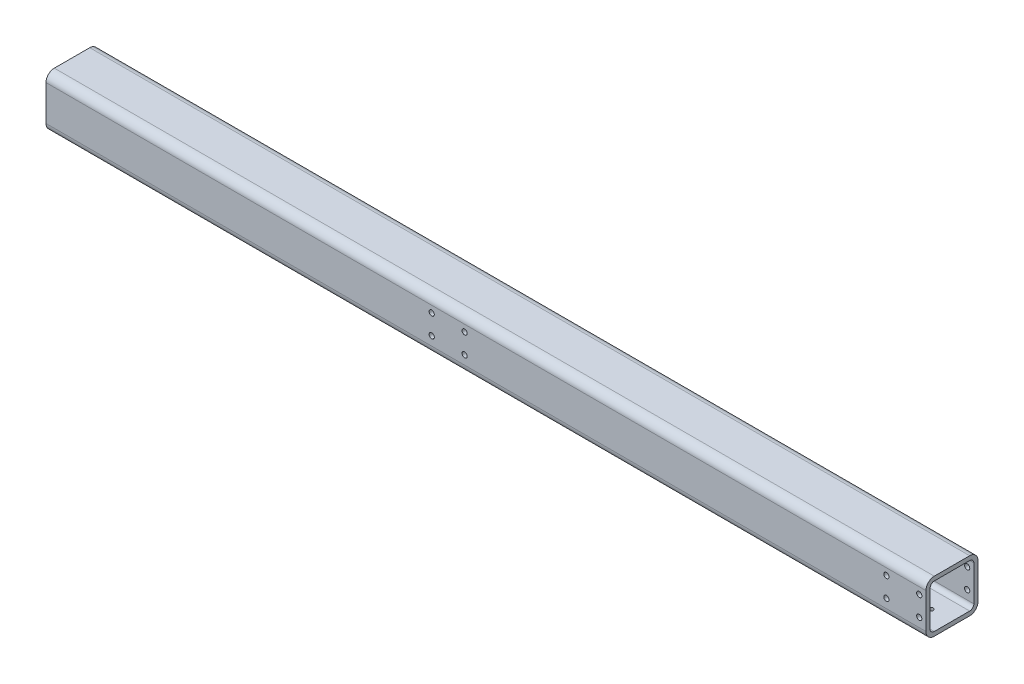
SolidWorks part; units mm, degrees
material "Q235A"
ref_plane "前视基准面" through (0, 0, 0) normal (0, 0, 1) x (1, 0, 0)
ref_plane "上视基准面" through (0, 0, 0) normal (0, 1, 0) x (1, 0, 0)
ref_plane "右视基准面" through (0, 0, 0) normal (1, 0, 0) x (0, 0, -1)
sketch "草图1" plane through (0, 0, 0) normal (0, 1, 0) x (1, 0, 0)
  line L0 (0, 0) -> (-845, 0)
  dimension "D1" = 845
other "Gb／6728-1986方形空心型钢 050 X 50 X 4(1)"
ref_plane "基准面1" through (0, 0, 0) normal (-1, 0, 0) x (0, 0, 1)
sketch "Sketch1" plane through (0, 0, 0) normal (-1, 0, 0) x (0, 0, 1)
  line L0 (-17, -21) -> (17, -21)
  line L1 (-21, -17) -> (-21, 17)
  line L2 (17, 21) -> (-17, 21)
  line L3 (21, 17) -> (21, -17)
  line L4 (-17, -25) -> (17, -25)
  line L5 (-25, -17) -> (-25, 17)
  line L6 (17, 25) -> (-17, 25)
  line L7 (25, 17) -> (25, -17)
  arc A0 (25, 17) -> (17, 25) centre (17, 17) ccw
  arc A1 (17, -25) -> (25, -17) centre (17, -17) ccw
  arc A2 (-25, -17) -> (-17, -25) centre (-17, -17) ccw
  arc A3 (-17, 25) -> (-25, 17) centre (-17, 17) ccw
  arc A4 (-17, 21) -> (-21, 17) centre (-17, 17) ccw
  arc A5 (21, 17) -> (17, 21) centre (17, 17) ccw
  arc A6 (17, -21) -> (21, -17) centre (17, -17) ccw
  arc A7 (-21, -17) -> (-17, -21) centre (-17, -17) ccw
  point P0 (-25, 0)
  point P1 (25, 0)
  point P2 (0, 25)
  point P3 (0, -25)
  point P4 (0, 0)
  point P5 (-25, -25)
  point P6 (25, -25)
  point P7 (25, 25)
  point P8 (-25, 25)
  point P33 (0, 0)
  dimension "D1" = 8
  dimension "Thickness" = 4
  dimension "V_leg" = 50
sketch "草图6" plane through (-845, 0, 0) normal (-1, 0, 0) x (0, 0, 1)
  line L0 (21, -17) -> (21, 17) construction
  line L1 (-17, -21) -> (17, -21) construction
  line L2 (-21, 17) -> (-21, -17) construction
  line L3 (17, 21) -> (-17, 21) construction
  line L4 (21, -17) -> (21, 17)
  line L5 (-17, -21) -> (17, -21)
  line L6 (-21, 17) -> (-21, -17)
  line L7 (17, 21) -> (-17, 21)
  arc A0 (21, 17) -> (17, 21) centre (17, 17) ccw construction
  arc A1 (17, -21) -> (21, -17) centre (17, -17) ccw construction
  arc A2 (-21, -17) -> (-17, -21) centre (-17, -17) ccw construction
  arc A3 (-17, 21) -> (-21, 17) centre (-17, 17) ccw construction
  arc A4 (21, 17) -> (17, 21) centre (17, 17) ccw
  arc A5 (17, -21) -> (21, -17) centre (17, -17) ccw
  arc A6 (-21, -17) -> (-17, -21) centre (-17, -17) ccw
  arc A7 (-17, 21) -> (-21, 17) centre (-17, 17) ccw
extrude "凸台-拉伸1" [suppressed] add sketch "草图6" against normal blind 10 separate body
hole_wizard "M6 螺纹孔1" positions "草图7" profile "草图8" tap size "M6" standard "ISO" end condition through all
sketch "草图7" plane through (0, 0, -25) normal (0, 0, -1) x (-1, 0, 0)
  line L0 (38, -8.4) -> (474.6, -8.4) construction
  line L1 (0, 17) -> (0, -17) construction
  line L3 (845, -25) -> (0, -25) construction
  point P0 (6.4, 10.6)
  point P3 (6.4, -8.4)
  point P6 (38, 10.6)
  point P9 (38, -8.4)
  point P16 (443, 10.6)
  point P17 (443, -8.4)
  point P18 (474.6, 10.6)
  point P19 (474.6, -8.4)
  dimension "D1" = 2
  dimension "D2" = 436.6
  dimension "D3" = 6.4
  dimension "D4" = 38
  dimension "D5" = 19
  dimension "D6" = 16.6
sketch "草图8" plane through (-6.4, 10.6, -25) normal (1, 0, 0) x (0, 1, 0)
  line L0 (0, 0) -> (0, 50)
  line L1 (0, 50) -> (2.5, 50)
  line L2 (2.5, 50) -> (2.5, 0)
  line L5 (2.5, 0) -> (0, 0)
  line L11 (0, -6.35) -> (0, 107.95) construction
  dimension "通孔螺纹孔钻头直径" = 5
  dimension "通孔螺纹孔钻头深度" = 50
cosmetic thread "孔螺蚊线1" parameters "D2"=6
cosmetic thread "孔螺蚊线2" parameters "D2"=6
cosmetic thread "孔螺蚊线3" parameters "D2"=6
cosmetic thread "孔螺蚊线4" parameters "D2"=6
cosmetic thread "孔螺蚊线5" parameters "D2"=6
cosmetic thread "孔螺蚊线6" parameters "D2"=6
cosmetic thread "孔螺蚊线7" parameters "D2"=6
cosmetic thread "孔螺蚊线8" parameters "D2"=6
hole_wizard "M5 螺纹孔1" positions "草图9" profile "草图10" tap size "M5" standard "ISO"
sketch "草图9" plane through (0, -25, 0) normal (0, -1, 0) x (-1, 0, 0)
  line L0 (0, 0) -> (20, 0)
  line L2 (20, 0) -> (190, 0) construction
  point P0 (20, 0)
  point P11 (190, 0)
  point P12 (360, 0)
  point P13 (530, 0)
  dimension "D1" = 20
  dimension "D3" = 170
  dimension "D2" = 4
sketch "草图10" plane through (-20, -25, 0) normal (1, 0, 0) x (0, 0, -1)
  line L0 (0, 0) -> (0, 4)
  line L1 (0, 4) -> (2.1, 4)
  line L2 (2.1, 4) -> (2.1, 0)
  line L5 (2.1, 0) -> (0, 0)
  line L11 (0, -6.35) -> (0, 107.95) construction
  dimension "通孔螺纹孔钻头直径" = 4.2
  dimension "通孔螺纹孔钻头深度" = 4
cosmetic thread "孔螺蚊线9" parameters "D2"=5
cosmetic thread "孔螺蚊线10" parameters "D2"=5
cosmetic thread "孔螺蚊线11" parameters "D2"=5
cosmetic thread "孔螺蚊线12" parameters "D2"=5
